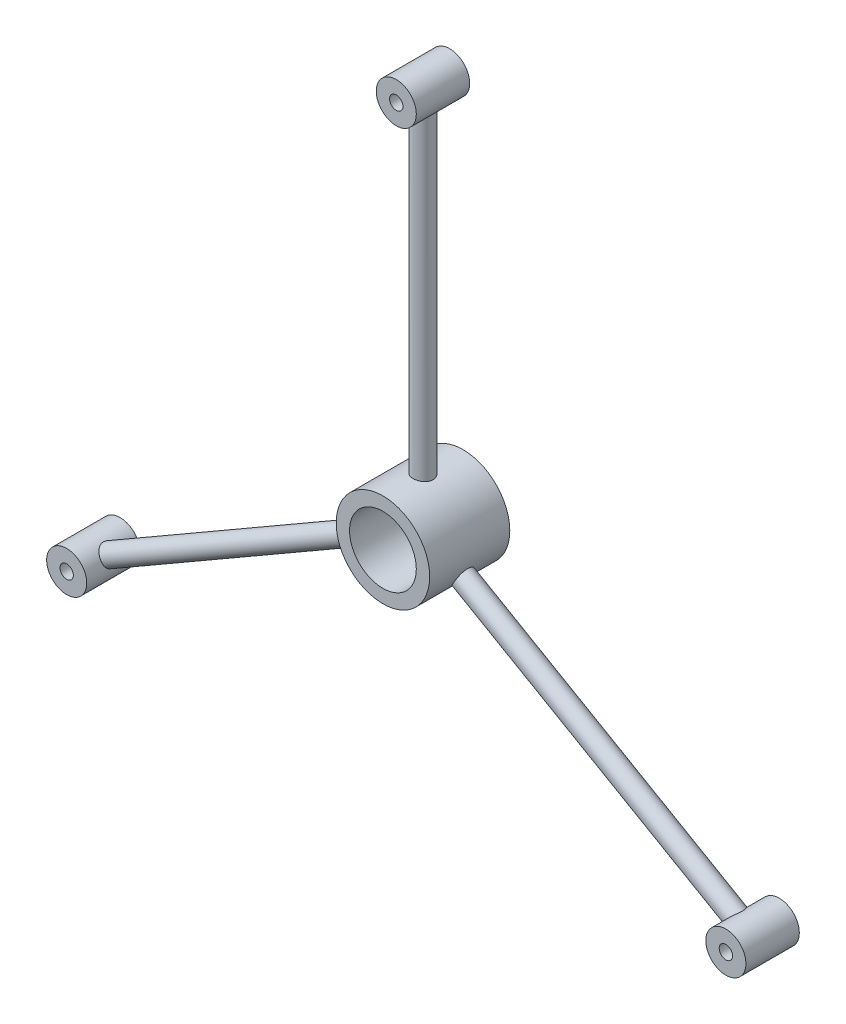
from build123d import *

# Parameters (mm, degrees)
SKETCH1_R           = 35
SKETCH1_R_2         = 25
BOSS_EXTRUDE1_DEPTH = 30
SKETCH3_R           = 7.5
BOSS_EXTRUDE2_DEPTH = 251
SKETCH4_R           = 15
SKETCH4_R_2         = 5
BOSS_EXTRUDE3_DEPTH = 20
CIRPATTERN3_COUNT   = 3


with BuildPart() as part:
    # Sketch1 → Boss-Extrude1 (new, symmetric)
    with BuildSketch(Plane.XY):
        Circle(SKETCH1_R)
        Circle(SKETCH1_R_2, mode=Mode.SUBTRACT)
    extrude(amount=BOSS_EXTRUDE1_DEPTH, both=True)


with BuildPart() as body_2:
    # Sketch3 → Boss-Extrude2 (new body)
    with BuildSketch(Plane(origin=(0, 25, 0), x_dir=(1, 0, 0), z_dir=(0, 1, 0))):
        with Locations(Location((0, 0, 0), (0, 0, 270))):
            Circle(SKETCH3_R)
    boss_extrude2 = extrude(amount=BOSS_EXTRUDE2_DEPTH)

    # Sketch4 → Boss-Extrude3 (add, symmetric)
    with BuildSketch(Plane.XY):
        with Locations((0, 285)):
            Circle(SKETCH4_R)
        with Locations((0, 285)):
            Circle(SKETCH4_R_2, mode=Mode.SUBTRACT)
    boss_extrude3 = extrude(amount=BOSS_EXTRUDE3_DEPTH, both=True)


with BuildPart() as part_1:
    add(part.part)

    # CirPattern3: Boss-Extrude2, Boss-Extrude3 ×3 about axis
    cirpattern3_axis = Axis((0, 0, 0), (0, 0, 1))
    add([boss_extrude2.rotate(cirpattern3_axis, i * 360 / CIRPATTERN3_COUNT) for i in range(1, CIRPATTERN3_COUNT)])
    add([boss_extrude3.rotate(cirpattern3_axis, i * 360 / CIRPATTERN3_COUNT) for i in range(1, CIRPATTERN3_COUNT)])


solid = Compound([body_2.part, part_1.part])
